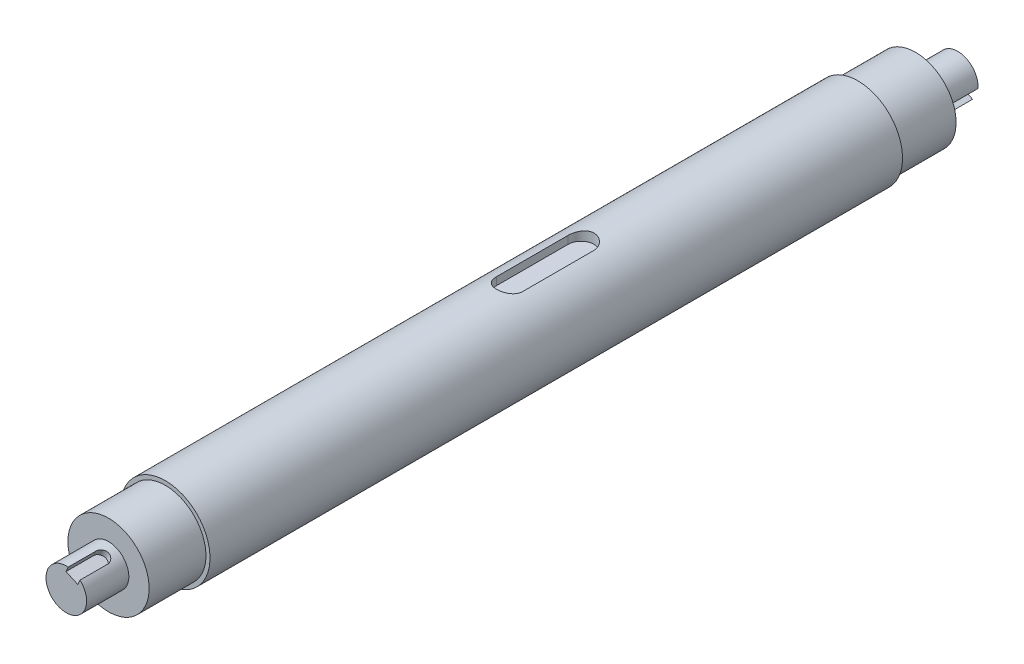
from build123d import *

# Parameters (mm, degrees)
CUT_EXTRUDE_3_DEPTH = 6
CUT_EXTRUDE_4_DEPTH = 7.3
CUT_EXTRUDE_5_DEPTH = 7.3


with BuildPart() as part:
    # 草图1 → 旋转1 (revolve)
    with BuildSketch(Plane(origin=(0, 0, 0), x_dir=(1, 0, 0), z_dir=(0, 1, 0))):
        Polygon((0, 100), (-12.5, 100), (-12.5, 74), (-25, 74), (-25, 38.53), (-27.5, 38.53), (-27.5, -387.93), (-25, -387.93), (-25, -422.93), (-12.5, -422.93), (-12.5, -448.93), (0, -448.93), align=None)
    revolve(axis=Axis((0, 0, 0), (0, 0, 1)))

    # 草图6 → 切除-拉伸3 (cut)
    with BuildSketch(Plane(origin=(0, 27.5, 0), x_dir=(1, 0, 0), z_dir=(0, 1, 0))):
        with BuildLine():
            Line((8, -131.93), (8, -175.93))
            ThreePointArc((8, -175.93), (0, -183.93), (-8, -175.93))
            Line((-8, -175.93), (-8, -131.93))
            ThreePointArc((-8, -131.93), (0, -123.93), (8, -131.93))
        make_face()
    extrude(amount=-CUT_EXTRUDE_3_DEPTH, mode=Mode.SUBTRACT)

    # 草图7 → 切除-拉伸4 (cut)
    with BuildSketch(Plane(origin=(14.434018231, -6.426438961, 0), x_dir=(0, 0, 1), z_dir=(-0.9135454576427331, 0.40673664307550317, 0))):
        with BuildLine():
            Line((-105.847779708, 4), (-83, 4))
            ThreePointArc((-83, 4), (-79, 0), (-83, -4))
            Line((-83, -4), (-105.847779708, -4))
            ThreePointArc((-105.847779708, -4), (-109.847779708, 0), (-105.847779708, 4))
        make_face()
    extrude(amount=CUT_EXTRUDE_4_DEPTH, mode=Mode.SUBTRACT)

    # 草图8 → 切除-拉伸5 (cut)
    with BuildSketch(Plane(origin=(6.426438961, 14.434018231, 0), x_dir=(0, 0, 1), z_dir=(-0.40673664307579893, -0.9135454576426014, 0))):
        with BuildLine():
            Line((455.303918894, -4), (431.93, -4))
            ThreePointArc((431.93, -4), (427.93, 0), (431.93, 4))
            Line((431.93, 4), (455.303918894, 4))
            ThreePointArc((455.303918894, 4), (459.303918894, 0), (455.303918894, -4))
        make_face()
    extrude(amount=CUT_EXTRUDE_5_DEPTH, mode=Mode.SUBTRACT)


solid = part.part
